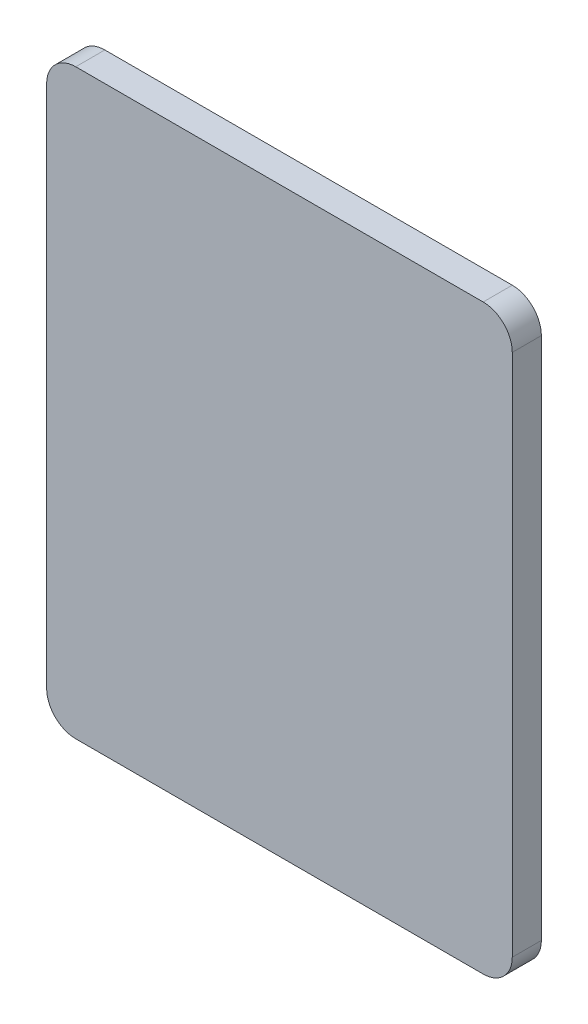
from build123d import *

# Parameters (mm, degrees)
SKETCH1_W           = 80
SKETCH1_H           = 100
BOSS_EXTRUDE1_DEPTH = 5
FILLET1_R           = 5


with BuildPart() as part:
    # Sketch1 → Boss-Extrude1 (new body)
    with BuildSketch(Plane.XY):
        with Locations((40, -50)):
            Rectangle(SKETCH1_W, SKETCH1_H)
    extrude(amount=BOSS_EXTRUDE1_DEPTH)

    # Fillet1
    fillet1_edges = [part.edges().sort_by_distance(p)[0] for p in [
        (0, 0, 2.5),
        (80, 0, 2.5),
        (80, -100, 2.5),
        (0, -100, 2.5),
    ]]
    fillet(fillet1_edges, radius=FILLET1_R)


solid = part.part
